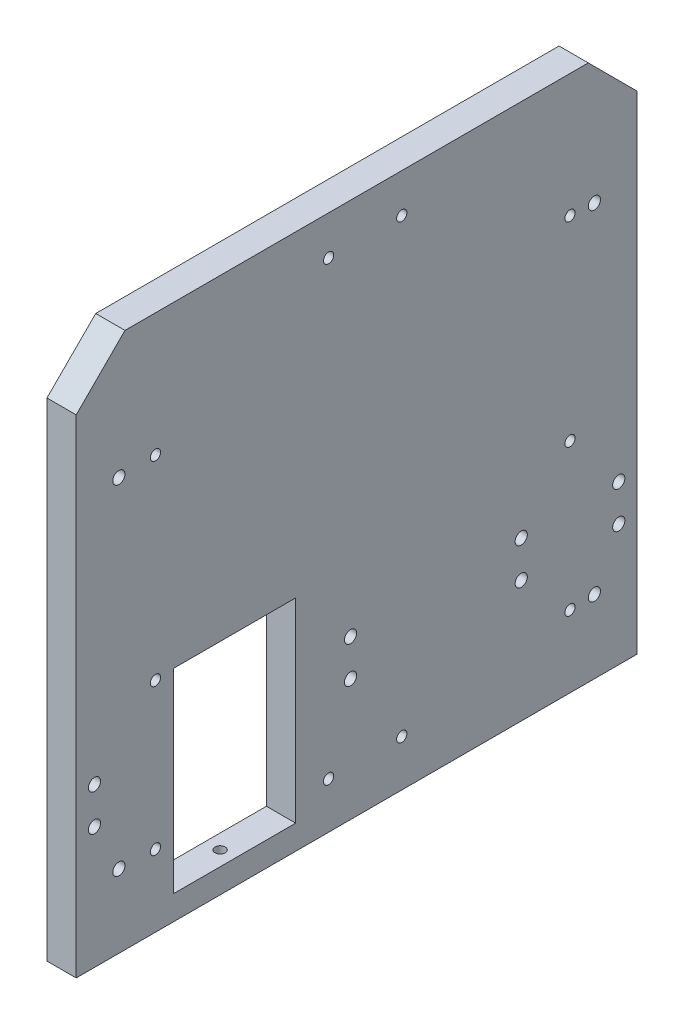
from build123d import *

# Parameters (mm, degrees)
SKETCH_1_W                  = 230
SKETCH_1_H                  = 220
BOSS_EXTRUDE_1_DEPTH        = 12
CHAMFER_1_SIZE              = 20
SKETCH_11_W                 = 50
SKETCH_11_H                 = 80
CUT_EXTRUDE_1_DEPTH         = 160.590099944
M6_TAPPED_HOLE_1_D          = 5
LINEAR_PATTERN_4_COUNT      = 2
LINEAR_PATTERN_4_PITCH      = 15
LINEAR_PATTERN_5_COUNT      = 3
LINEAR_PATTERN_5_PITCH      = 50
LINEAR_PATTERN_5_COL_COUNT  = 3
LINEAR_PATTERN_5_COL_PITCH  = 50
LINEAR_PATTERN_6_COUNT      = 2
LINEAR_PATTERN_6_PITCH      = 110
LINEAR_PATTERN_6_COPY_1_D   = 5
M5_TAPPED_HOLE_2_D          = 4.2
LINEAR_PATTERN_7_COUNT      = 2
LINEAR_PATTERN_7_PITCH      = 30
LINEAR_PATTERN_7_COUNT_DIR2 = 2
LINEAR_PATTERN_7_PITCH_DIR2 = 185
LINEAR_PATTERN_8_COUNT      = 2
LINEAR_PATTERN_8_PITCH      = 139
LINEAR_PATTERN_9_COUNT      = 2
LINEAR_PATTERN_9_PITCH      = 195
M5_TAPPED_HOLE_3_D          = 4.2
LINEAR_PATTERN_10_COUNT     = 2
LINEAR_PATTERN_10_PITCH     = 60
LINEAR_PATTERN_11_COUNT     = 2
LINEAR_PATTERN_11_PITCH     = 140
LINEAR_PATTERN_12_COUNT     = 2
LINEAR_PATTERN_12_PITCH     = 170
LINEAR_PATTERN_12_COPY_1_D  = 4.2
LINEAR_PATTERN_12_COPY_2_D  = 4.2
LINEAR_PATTERN_13_COUNT     = 2
LINEAR_PATTERN_13_PITCH     = 215
LINEAR_PATTERN_13_COPY_1_D  = 5
LINEAR_PATTERN_14_COUNT     = 2
LINEAR_PATTERN_14_PITCH     = 40
LINEAR_PATTERN_14_COPY_1_D  = 5
LINEAR_PATTERN_15_COUNT     = 2
LINEAR_PATTERN_15_PITCH     = 10


with BuildPart() as part:
    # Sketch 1 → Boss-Extrude 1 (new body)
    with BuildSketch(Plane(origin=(0, 0, 0), x_dir=(0, 0, -1), z_dir=(1, 0, 0))):
        Rectangle(SKETCH_1_W, SKETCH_1_H)
    extrude(amount=BOSS_EXTRUDE_1_DEPTH)

    # Chamfer 1
    chamfer_1_edges = [part.edges().sort_by_distance(p)[0] for p in [
        (6, 110, 115),
        (6, 110, -115),
    ]]
    chamfer(chamfer_1_edges, length=CHAMFER_1_SIZE)

    # Sketch 11 → Cut-Extrude 1 (cut, through all)
    with BuildSketch(Plane.ZY):
        with Locations((50, -60)):
            Rectangle(SKETCH_11_W, SKETCH_11_H)
    extrude(amount=-CUT_EXTRUDE_1_DEPTH, mode=Mode.SUBTRACT)

    # M6 Tapped Hole 1 (through all)
    with Locations(Plane.ZY):
        with Locations((-107.5, -60)):
            m6_tapped_hole_1 = Hole(M6_TAPPED_HOLE_1_D / 2)

    # Linear Pattern 4: M6 Tapped Hole 1 ×2
    with Locations(*[(0, i * LINEAR_PATTERN_4_PITCH, 0) for i in range(1, LINEAR_PATTERN_4_COUNT)]):
        add(m6_tapped_hole_1, mode=Mode.SUBTRACT)

    # Sketch 14 → M5 Tapped Hole 1 (revolve, cut)
    with BuildSketch(Plane(origin=(6, -110, 0), x_dir=(0, 0, -1), z_dir=(1, 0, 0))):
        Polygon((0, 0), (0, 13.6618073), (2.1, 12.4), (2.1, 0), align=None)
    m5_tapped_hole_1 = revolve(axis=Axis((6, -116.35, 0), (0, 1, 0)), mode=Mode.SUBTRACT)

    # Linear Pattern 5: M5 Tapped Hole 1 ×3
    with Locations(*[(0, 0, -i * LINEAR_PATTERN_5_PITCH) for i in range(1, LINEAR_PATTERN_5_COUNT)]):
        add(m5_tapped_hole_1, mode=Mode.SUBTRACT)

    # Linear Pattern 5 col: M5 Tapped Hole 1 ×3
    with Locations(*[(0, 0, i * LINEAR_PATTERN_5_COL_PITCH) for i in range(1, LINEAR_PATTERN_5_COL_COUNT)]):
        add(m5_tapped_hole_1, mode=Mode.SUBTRACT)

    # Linear Pattern 6: M6 Tapped Hole 1 ×2
    with Locations(*[(0, 0, i * LINEAR_PATTERN_6_PITCH) for i in range(1, LINEAR_PATTERN_6_COUNT)]):
        add(m6_tapped_hole_1, mode=Mode.SUBTRACT)

    # Linear Pattern 6 copy 1 (through all)
    with Locations(Plane(origin=(0, 15, 110), x_dir=(0, 0, 1), z_dir=(-1, 0, 0))):
        with Locations((-107.5, -60)):
            Hole(LINEAR_PATTERN_6_COPY_1_D / 2)

    # M5 Tapped Hole 2 (through all)
    with Locations(Plane.ZY):
        with Locations((11.5, -91)):
            m5_tapped_hole_2 = Hole(M5_TAPPED_HOLE_2_D / 2)

    # Linear Pattern 7: M5 Tapped Hole 2 2 × 2
    with Locations(*[(0, j * LINEAR_PATTERN_7_PITCH_DIR2, -i * LINEAR_PATTERN_7_PITCH) for i in range(LINEAR_PATTERN_7_COUNT) for j in range(LINEAR_PATTERN_7_COUNT_DIR2) if (i, j) != (0, 0)]):
        add(m5_tapped_hole_2, mode=Mode.SUBTRACT)

    # Sketch 18 → Ø5.0 (5) Hole 1 (revolve, cut)
    with BuildSketch(Plane(origin=(12, -80, 97.5), x_dir=(0, 0, -1), z_dir=(0, 1, 0))):
        Polygon((0, 0), (0, 21.502151548), (2.5, 20), (2.5, 0), align=None)
    f_5_0_5_hole_1 = revolve(axis=Axis((18.35, -80, 97.5), (-1, 0, 0)), mode=Mode.SUBTRACT)

    # Linear Pattern 8: Ø5.0 (5) Hole 1 ×2
    with Locations(*[(0, i * LINEAR_PATTERN_8_PITCH, 0) for i in range(1, LINEAR_PATTERN_8_COUNT)]):
        add(f_5_0_5_hole_1, mode=Mode.SUBTRACT)

    # Linear Pattern 9: Ø5.0 (5) Hole 1 ×2
    with Locations(*[(0, 0, -i * LINEAR_PATTERN_9_PITCH) for i in range(1, LINEAR_PATTERN_9_COUNT)]):
        add(f_5_0_5_hole_1, mode=Mode.SUBTRACT)

    # Linear Pattern 9 copy 1 sketch → Linear Pattern 9 copy 1 (revolve, cut)
    with BuildSketch(Plane(origin=(12, 59, -97.5), x_dir=(0, 0, -1), z_dir=(0, 1, 0))):
        Polygon((0, 0), (0, 21.502151548), (2.5, 20), (2.5, 0), align=None)
    revolve(axis=Axis((18.35, 59, -97.5), (-1, 0, 0)), mode=Mode.SUBTRACT)

    # M5 Tapped Hole 3 (through all)
    with Locations(Plane(origin=(12, 0, 0), x_dir=(0, 0, -1), z_dir=(1, 0, 0))):
        with Locations((-82.5, -80.5)):
            m5_tapped_hole_3 = Hole(M5_TAPPED_HOLE_3_D / 2)

    # Linear Pattern 10: M5 Tapped Hole 3 ×2
    with Locations(*[(0, i * LINEAR_PATTERN_10_PITCH, 0) for i in range(1, LINEAR_PATTERN_10_COUNT)]):
        add(m5_tapped_hole_3, mode=Mode.SUBTRACT)

    # Linear Pattern 11: M5 Tapped Hole 3 ×2
    with Locations(*[(0, i * LINEAR_PATTERN_11_PITCH, 0) for i in range(1, LINEAR_PATTERN_11_COUNT)]):
        add(m5_tapped_hole_3, mode=Mode.SUBTRACT)

    # Linear Pattern 12: M5 Tapped Hole 3 ×2
    with Locations(*[(0, 0, -i * LINEAR_PATTERN_12_PITCH) for i in range(1, LINEAR_PATTERN_12_COUNT)]):
        add(m5_tapped_hole_3, mode=Mode.SUBTRACT)

    # Linear Pattern 12 copy 1 (through all)
    with Locations(Plane(origin=(12, 60, -170), x_dir=(0, 0, -1), z_dir=(1, 0, 0))):
        with Locations((-82.5, -80.5)):
            Hole(LINEAR_PATTERN_12_COPY_1_D / 2)

    # Linear Pattern 12 copy 2 (through all)
    with Locations(Plane(origin=(12, 140, -170), x_dir=(0, 0, -1), z_dir=(1, 0, 0))):
        with Locations((-82.5, -80.5)):
            Hole(LINEAR_PATTERN_12_COPY_2_D / 2)

    # Linear Pattern 13: M6 Tapped Hole 1 ×2
    with Locations(*[(0, 0, i * LINEAR_PATTERN_13_PITCH) for i in range(1, LINEAR_PATTERN_13_COUNT)]):
        add(m6_tapped_hole_1, mode=Mode.SUBTRACT)

    # Linear Pattern 13 copy 1 (through all)
    with Locations(Plane(origin=(0, 15, 215), x_dir=(0, 0, 1), z_dir=(-1, 0, 0))):
        with Locations((-107.5, -60)):
            Hole(LINEAR_PATTERN_13_COPY_1_D / 2)

    # Linear Pattern 14: M6 Tapped Hole 1 ×2
    with Locations(*[(0, 0, i * LINEAR_PATTERN_14_PITCH) for i in range(1, LINEAR_PATTERN_14_COUNT)]):
        add(m6_tapped_hole_1, mode=Mode.SUBTRACT)

    # Linear Pattern 14 copy 1 (through all)
    with Locations(Plane(origin=(0, 15, 40), x_dir=(0, 0, 1), z_dir=(-1, 0, 0))):
        with Locations((-107.5, -60)):
            Hole(LINEAR_PATTERN_14_COPY_1_D / 2)

    # Sketch 22 → M3 Tapped Hole 1 (revolve, cut)
    with BuildSketch(Plane(origin=(0, -70, -110), x_dir=(0, 0, 1), z_dir=(0, 1, 0))):
        Polygon((0, 0), (0, 8.251075774), (1.25, 7.5), (1.25, 0), align=None)
    m3_tapped_hole_1 = revolve(axis=Axis((-6.35, -70, -110), (1, 0, 0)), mode=Mode.SUBTRACT)

    # Linear Pattern 15: M3 Tapped Hole 1 ×2
    with Locations(*[(0, -i * LINEAR_PATTERN_15_PITCH, 0) for i in range(1, LINEAR_PATTERN_15_COUNT)]):
        add(m3_tapped_hole_1, mode=Mode.SUBTRACT)


solid = part.part
